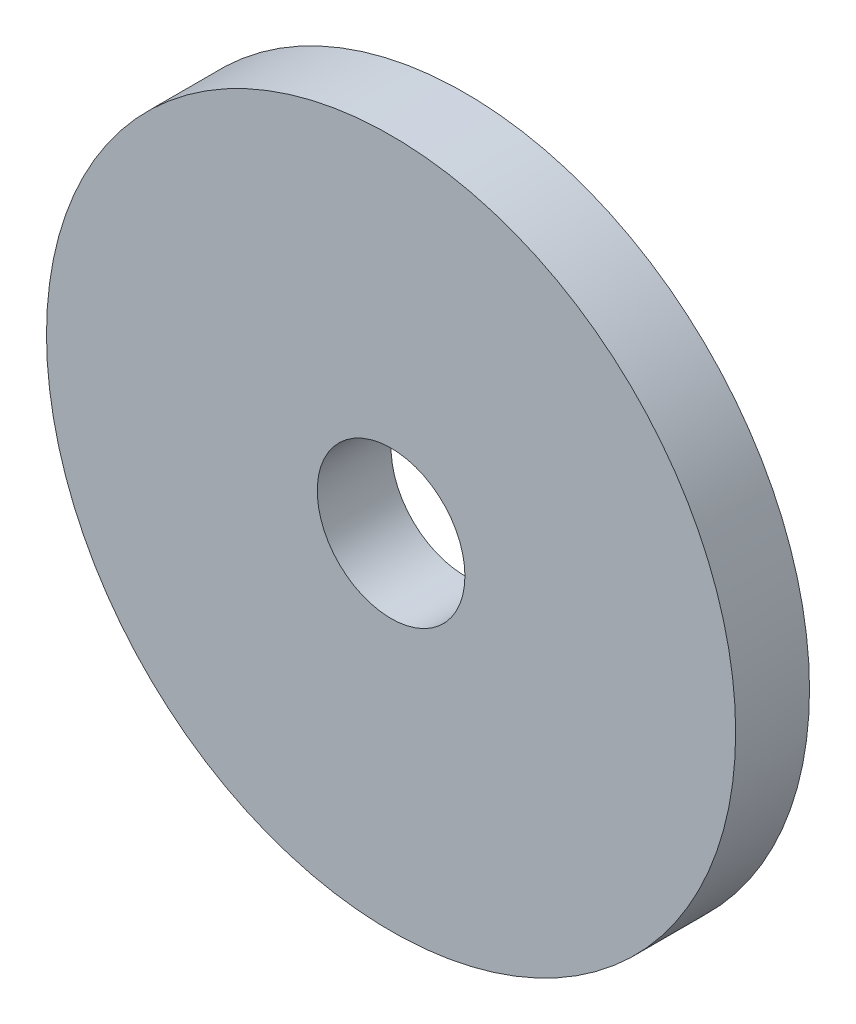
SolidWorks part; units mm, degrees
ref_plane "Front Plane" through (0, 0, 0) normal (0, 0, 1) x (1, 0, 0)
ref_plane "Top Plane" through (0, 0, 0) normal (0, 1, 0) x (1, 0, 0)
ref_plane "Right Plane" through (0, 0, 0) normal (1, 0, 0) x (0, 0, -1)
sketch "Sketch1" plane through (0, 0, 0) normal (0, 0, 1) x (1, 0, 0)
  circle A0 centre (0, 0) radius 3
  circle A1 centre (0, 0) radius 14
  dimension "D1" = 6
  dimension "D2" = 28
extrude "Boss-Extrude1" add sketch "Sketch1" along normal blind 3
